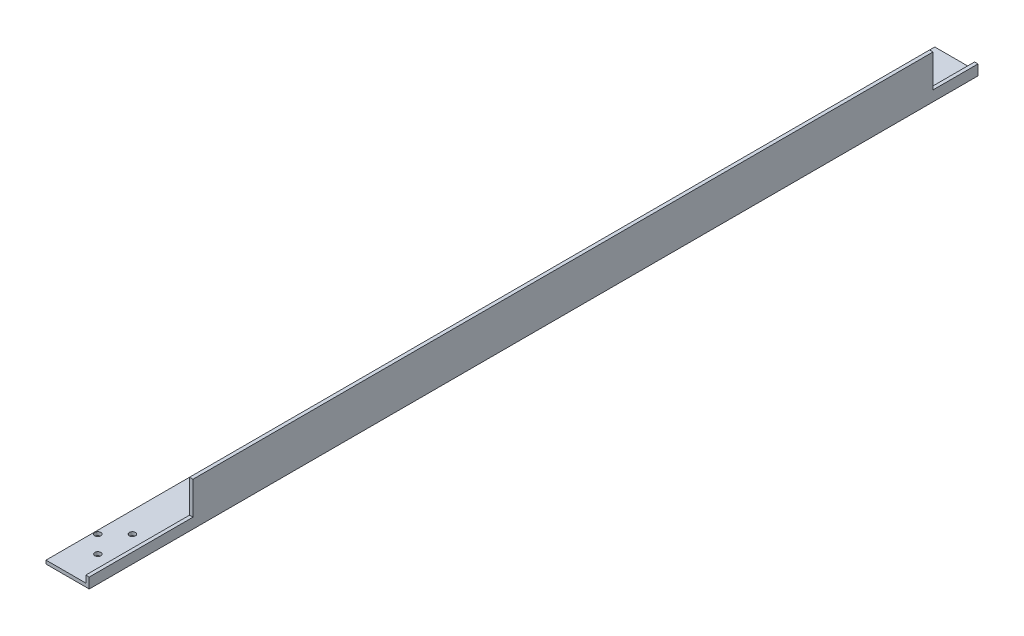
SolidWorks part; units mm, degrees
material "A3"
ref_plane "前视基准面" through (0, 0, 0) normal (0, 0, 1) x (1, 0, 0)
ref_plane "上视基准面" through (0, 0, 0) normal (0, 1, 0) x (1, 0, 0)
ref_plane "右视基准面" through (0, 0, 0) normal (1, 0, 0) x (0, 0, -1)
sketch "草图1" plane through (0, 0, 0) normal (0, 0, 1) x (1, 0, 0)
  line L0 (-125, 0) -> (0, 0)
  line L1 (0, 0) -> (0, 125)
  line L2 (-125, 10) -> (-10, 10)
  line L3 (-10, 10) -> (-10, 125)
  line L4 (-125, 10) -> (-125, 0)
  line L5 (-10, 125) -> (0, 125)
  dimension "D1" = 125
  dimension "D2" = 10
extrude "凸台-拉伸1" add sketch "草图1" along normal mid plane 2570
hole_wizard "M20 螺纹孔1" positions "草图2" profile "草图3" tap size "M20" standard "GB" end condition through all
sketch "草图2" plane through (0, 10, 0) normal (0, 1, 0) x (1, 0, 0)
  line L0 (-100, 965) -> (-50, 965) construction
  line L1 (-100, 965) -> (-100, 1185) construction
  line L2 (0, -1285) -> (0, 1285) construction
  line L3 (-115, -1145) -> (0, -1145) construction
  line L5 (0, 125) -> (-125, 125) construction
  line L6 (-125, -1285) -> (-125, 1285) construction
  line L8 (-10, 1285) -> (-125, 1285) construction
  point P0 (-100, 965)
  point P6 (-50, 965)
  point P7 (-50, 1185)
  point P8 (-100, 1185)
  point P14 (-100, 1075)
  point P16 (-115, -1145)
  point P18 (-65, -1095)
  point P26 (-65, -1195)
  dimension "D2" = 50
  dimension "D3" = 220
  dimension "D5" = 50
  dimension "D6" = 950
  dimension "D7" = 1270
  dimension "D8" = 115
  dimension "D9" = 50
  dimension "D10" = 65
  dimension "D11" = 100
  dimension "D4" = 2
  dimension "D1" = 2
sketch "草图3" plane through (-100, 10, -965) normal (1, 0, 0) x (0, 0, 1)
  line L0 (0, 0) -> (0, 10)
  line L1 (0, 10) -> (8.75, 10)
  line L2 (8.75, 10) -> (8.75, 0)
  line L5 (8.75, 0) -> (0, 0)
  line L11 (0, -6.35) -> (0, 107.95) construction
  dimension "通孔螺纹孔钻头直径" = 17.5
  dimension "通孔螺纹孔钻头深度" = 10
cosmetic thread "孔螺蚊线1"
cosmetic thread "孔螺蚊线2"
cosmetic thread "孔螺蚊线3"
cosmetic thread "孔螺蚊线4"
cosmetic thread "孔螺蚊线5"
cosmetic thread "孔螺蚊线6"
cosmetic thread "孔螺蚊线7"
sketch "草图4" plane through (-10, 0, 0) normal (-1, 0, 0) x (0, 0, 1)
  line L1 (1285, 125) -> (985, 125)
  line L2 (1285, 125) -> (1285, 30)
  line L3 (1285, 30) -> (985, 30)
  line L4 (985, 125) -> (985, 30)
  line L5 (-1285, 125) -> (-1155, 125)
  line L6 (-1285, 125) -> (-1285, 30)
  line L7 (-1285, 30) -> (-1155, 30)
  line L8 (-1155, 125) -> (-1155, 30)
  dimension "D1" = 95
  dimension "D2" = 300
  dimension "D3" = 130
extrude "切除-拉伸1" cut sketch "草图4" against normal through all
